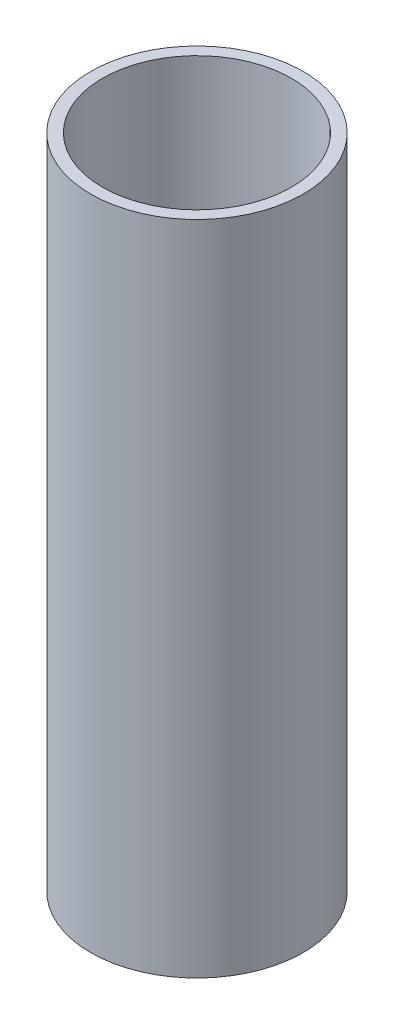
from build123d import *

# Parameters (mm, degrees)
SKETCH1_R           = 450
SKETCH1_R_2         = 400
BOSS_EXTRUDE1_DEPTH = 1650
MOVE_FACE1_BY       = 518


with BuildPart() as part:
    # Sketch1 → Boss-Extrude1 (new, symmetric)
    with BuildSketch(Plane(origin=(0, 0, 0), x_dir=(1, 0, 0), z_dir=(0, 1, 0))):
        with Locations(Location((0, 0, 0), (0, 0, 270))):
            Circle(SKETCH1_R)
        with Locations(Location((0, 0, 0), (0, 0, 270))):
            Circle(SKETCH1_R_2, mode=Mode.SUBTRACT)
    extrude(amount=BOSS_EXTRUDE1_DEPTH, both=True)

    # Move Face1: a face moved inward by 518.0
    extrude(part.faces().sort_by_distance((-225, -1650, 360))[0], amount=MOVE_FACE1_BY, dir=(0, 1, 0), mode=Mode.SUBTRACT)


solid = part.part
